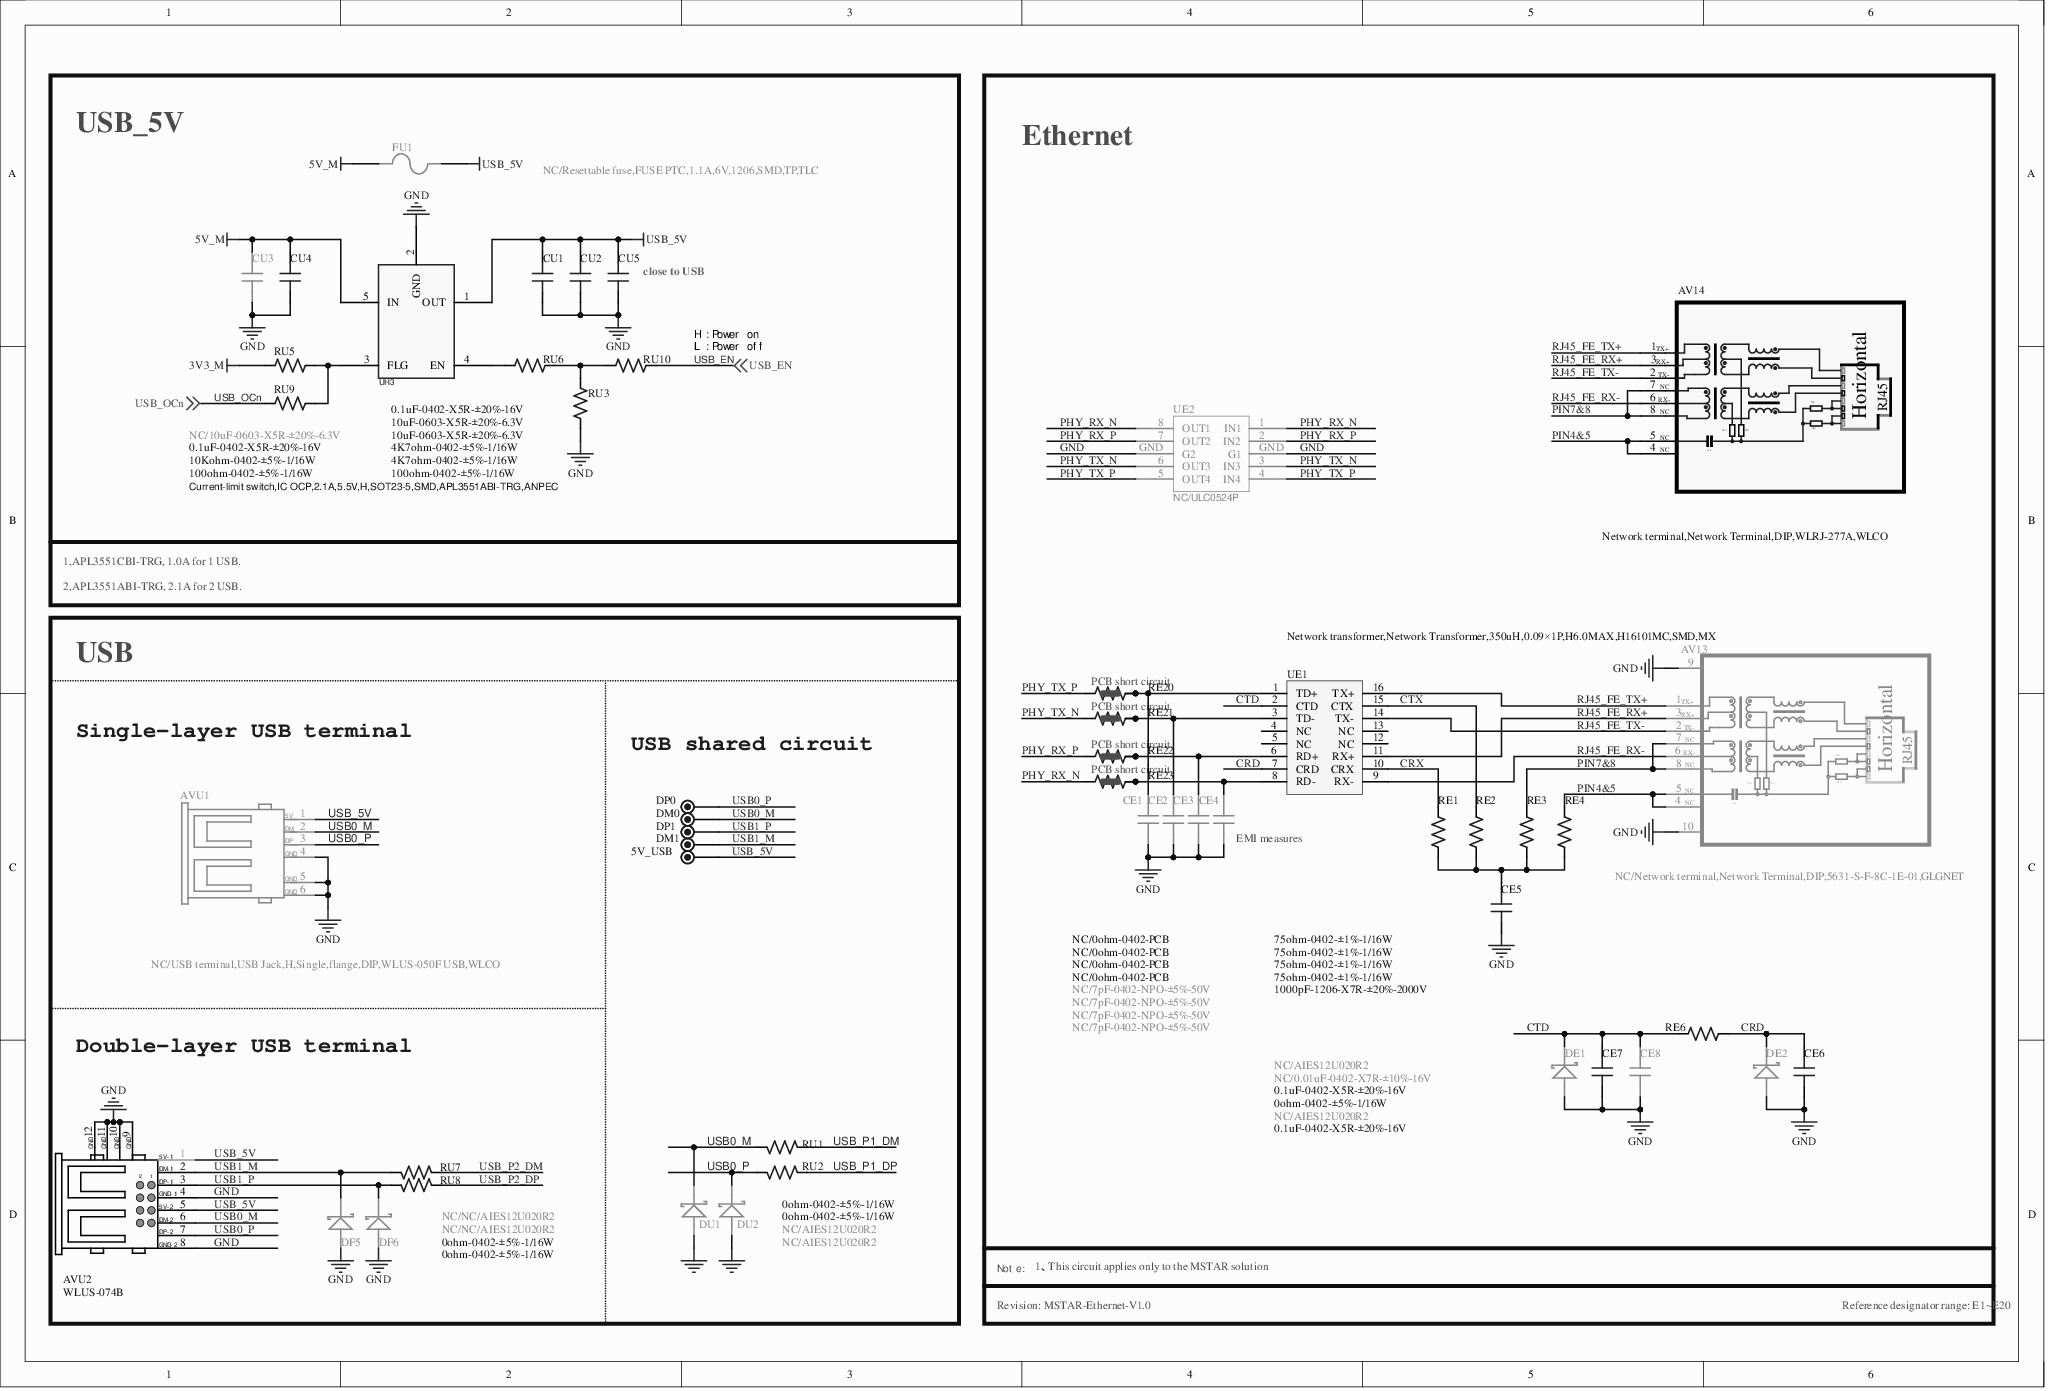
[diagram p0: MISC86290-16.SchDoc]
# Altium project MISC86290.PrjPcb (part 12 of 13)

## Sheet MISC86290-16.SchDoc
size 411 x 279 mm

### Parts
5V_USB  TEST  [TP]  (value not drawn)
AV13  NC/Network terminal,Network Terminal,DIP,5631-S-F-8C-1E-01,GLGNET  [RJ45U-D-5]
AV14  Network terminal,Network Terminal,DIP,WLRJ-277A,WLCO  [RJ45U-D-14]
AVU1  NC/USB terminal,USB Jack,H,Single,flange,DIP,WLUS-050F USB,WLCO  [USB1-HD-2]
AVU2  WLUS-074B  [USB2-HD-1]
CE1  NC/7pF-0402-NPO-±5%-50V  [C0402]
CE2  NC/7pF-0402-NPO-±5%-50V  [C0402]
CE3  NC/7pF-0402-NPO-±5%-50V  [C0402]
CE4  NC/7pF-0402-NPO-±5%-50V  [C0402]
CE5  1000pF-1206-X7R-±20%-2000V  [C1206]
CE6  0.1uF-0402-X5R-±20%-16V  [C0402]
CE7  0.1uF-0402-X5R-±20%-16V  [C0402]
CE8  NC/0.01uF-0402-X7R-±10%-16V  [C0402]
CU1  0.1uF-0402-X5R-±20%-16V  [C0402]
CU2  10uF-0603-X5R-±20%-6.3V  [C0603]
CU3  NC/10uF-0603-X5R-±20%-6.3V  [C0603]
CU4  0.1uF-0402-X5R-±20%-16V  [C0402]
CU5  10uF-0603-X5R-±20%-6.3V  [C0603]
DE1  NC/AIES12U020R2  [DIODE-S0402]
DE2  NC/AIES12U020R2  [DIODE-S0402]
DF5  NC/NC/AIES12U020R2  [DIODE-S0402]
DF6  NC/NC/AIES12U020R2  [DIODE-S0402]
DM0  TEST  [TP]  (value not drawn)
DM1  TEST  [TP]  (value not drawn)
DP0  TEST  [TP]  (value not drawn)
DP1  TEST  [TP]  (value not drawn)
DU1  NC/AIES12U020R2  [DIODE-S0402]
DU2  NC/AIES12U020R2  [DIODE-S0402]
FU1  NC/Resettable fuse,FUSE PTC,1.1A,6V,1206,SMD,TP,TLC  [FUSE1.1A-S]
RE1  75ohm-0402-±1%-1/16W  [R0402]
RE2  75ohm-0402-±1%-1/16W  [R0402]
RE3  75ohm-0402-±1%-1/16W  [R0402]
RE4  75ohm-0402-±1%-1/16W  [R0402]
RE6  0ohm-0402-±5%-1/16W  [R0402]
RE20  NC/0ohm-0402-PCB  [R0402SC]
RE21  NC/0ohm-0402-PCB  [R0402SC]
RE22  NC/0ohm-0402-PCB  [R0402SC]
RE23  NC/0ohm-0402-PCB  [R0402SC]
RU1  0ohm-0402-±5%-1/16W  [R0402]
RU2  0ohm-0402-±5%-1/16W  [R0402]
RU3  4K7ohm-0402-±5%-1/16W  [R0402]
RU5  10Kohm-0402-±5%-1/16W  [R0402]
RU6  4K7ohm-0402-±5%-1/16W  [R0402]
RU7  0ohm-0402-±5%-1/16W  [R0402]
RU8  0ohm-0402-±5%-1/16W  [R0402]
RU9  100ohm-0402-±5%-1/16W  [R0402]
RU10  100ohm-0402-±5%-1/16W  [R0402]
UE1  Network transformer,Network Transformer,350uH,0.09×1P,H6.0MAX,H16101MC,SMD,MX  [SOP16/1.27-2]
UE2  NC/ULC0524P  [RCL0524P]
UH3  Current-limit switch,IC OCP,2.1A,5.5V,H,SOT23-5,SMD,APL3551ABI-TRG,ANPEC  [SOT-23-5]

### Blocks framed on the sheet
USB_5V: CU1-CU5 FU1 RU3 RU5 RU6 RU9 RU10 UH3
Ethernet: AV13 AV14 CE1-CE8 DE1 DE2 RE1-RE4 RE6 RE20-RE23 UE1 UE2
USB: 5V_USB AVU1 AVU2 DF5 DF6 DM0 DM1 DP0 DP1 DU1 DU2 RU1 RU2 RU7 RU8

### Nets
3V3_M: RU5.1
5V_M: CU3.2 CU4.2 FU1.1 UH3.5(IN)
GND: AV13.9 AV13.10 AVU1.4 AVU1.5 AVU1.6 AVU2.4 AVU2.8 AVU2.9 AVU2.10 AVU2.11 AVU2.12 CE1.1 CE2.1 CE3.1 CE4.1 CE5.2 CE6.2 CE7.1 CE8.1 CU1.2 CU2.2 CU3.1 CU4.1 CU5.2 DE1.A DE2.A DF5.A DF6.A DU1.A DU2.A RU3.2 UE2.GND(G1) UH3.2(GND)
USB_5V: 5V_USB.1 AVU1.1 AVU2.1 AVU2.5 CU1.1 CU2.1 CU5.1 FU1.2 UH3.1(OUT)
CRD: CE6.1 DE2.K RE6.2 UE1.7(CRD)
CRX: RE1.2 UE1.10(CRX)
CTD: CE7.2 CE8.2 DE1.K RE6.1 UE1.2(CTD)
CTX: RE2.2 UE1.15(CTX)
PHY_RX_N: RE23.1 UE2.1(IN1) UE2.8(OUT1)
PHY_RX_P: RE22.1 UE2.2(IN2) UE2.7(OUT2)
PHY_TX_N: RE21.1 UE2.3(IN3) UE2.6(OUT3)
PHY_TX_P: RE20.1 UE2.4(IN4) UE2.5(OUT4)
PIN4&5: AV13.4 AV13.5 AV14.4 AV14.5 RE4.2
PIN7&8: AV13.7 AV13.8 AV14.7 AV14.8 RE3.2
RJ45_FE_RX+: AV13.3 AV14.3 UE1.11(RX+)
RJ45_FE_RX-: AV13.6 AV14.6 UE1.9(RX-)
RJ45_FE_TX+: AV13.1 AV14.1 UE1.16(TX+)
RJ45_FE_TX-: AV13.2 AV14.2 UE1.14(TX-)
USB0_M: AVU1.2 AVU2.6 DM0.1 DU1.K RU1.2
USB0_P: AVU1.3 AVU2.7 DP0.1 DU2.K RU2.2
USB1_M: AVU2.2 DF5.K DM1.1 RU7.2
USB1_P: AVU2.3 DF6.K DP1.1 RU8.2
USB_EN: RU10.2 ; off-sheet USB_EN
USB_OCn: RU9.1 ; off-sheet USB_OCn
USB_P1_DM: RU1.1
USB_P1_DP: RU2.1
USB_P2_DM: RU7.1
USB_P2_DP: RU8.1
NetCE1_2: CE1.2 RE20.2 RE20.3 UE1.1(TD+)
NetCE2_2: CE2.2 RE21.2 RE21.3 UE1.3(TD-)
NetCE3_2: CE3.2 RE22.2 RE22.3 UE1.6(RD+)
NetCE4_2: CE4.2 RE23.2 RE23.3 UE1.8(RD-)
NetCE5_1: CE5.1 RE1.1 RE2.1 RE3.1 RE4.1
NetRU3_1: RU3.1 RU6.1 RU10.1
NetRU5_2: RU5.2 RU9.2 UH3.3(FLG)
NetRU6_2: RU6.2 UH3.4(EN)

Not connected (* = marked no-connect by the designer): UE1 4(NC)* 5(NC)* 12(NC)* 13(NC)*

### Notes on the sheet
- (near CU5) close to USB
- H :Power on
- (near RU10) L :Power off
- 1,APL3551CBI-TRG, 1.0A for 1 USB.
- 2,APL3551ABI-TRG, 2.1A for 2 USB.
- Single-layer USB terminal
- USB shared circuit
- (near CE4) EMI measures
- Double-layer USB terminal
- Note:
- 1、This circuit applies only to the MSTAR solution
- Revision: MSTAR-Ethernet-V1.0
- Reference designator range: E1~E20

### Library data of the parts
AV13 = XXX.XXX.0002342: Network terminal,Network Terminal,DIP,5631-S-F-8C-1E-01,GLGNET-DLMI
AV14 = XXX.XXX.0002262: Network terminal,Network Terminal,DIP,41238-01G051,GLGNET-DLMI
AVU1 = USB-042M-002DP-DLMI-USB: CN-USB-#-#-#
AVU2 = USB-A/F-90°-DLMI-USB: CN-USB-double layer-#-#
CE1-CE4 = 7pF-0402-NPO-±5%-50V-D
CE5 = 1000pF-1206-X7R-±20%-2000V-D
CE6 CE7 CU1 = 0.1uF-0402-X5R-±20%-16V-D
CE8 = 0.01uF-0402-X7R-±10%-16V-D
CU2 CU3 CU5 = 10uF-0603-X5R-±20%-6.3V-D
CU4 = 0.1uF-0402-X7R-±10%-16V-D
DE1 DE2 DF5 DF6 DU1 DU2 = AIES12U020R2-D
FU1 = NSMD110(1206-1.1A)-D
RE1-RE4 = 75ohm-0402-±1%-1/16W-D
RE6 = 0ohm-0402-±5%-1/16W-D
RE20-RE23 = 0ohm-0402-PCB-D
RU1 RU2 RU7 RU8 = 5R1ohm-0402-±5%-1/16W-D
RU3 RU6 = 4K7ohm-0402-±5%-1/16W-D
RU5 RU9 RU10 = 10Kohm-0402-±5%-1/16W-D
UE1 = H16101MC-D
UE2 = ULC0524P-D: RCLAMP0524J
UH3 = AP2171WG-7-D

## Sheet MISC86290-17.SchDoc
size 406 x 325 mm
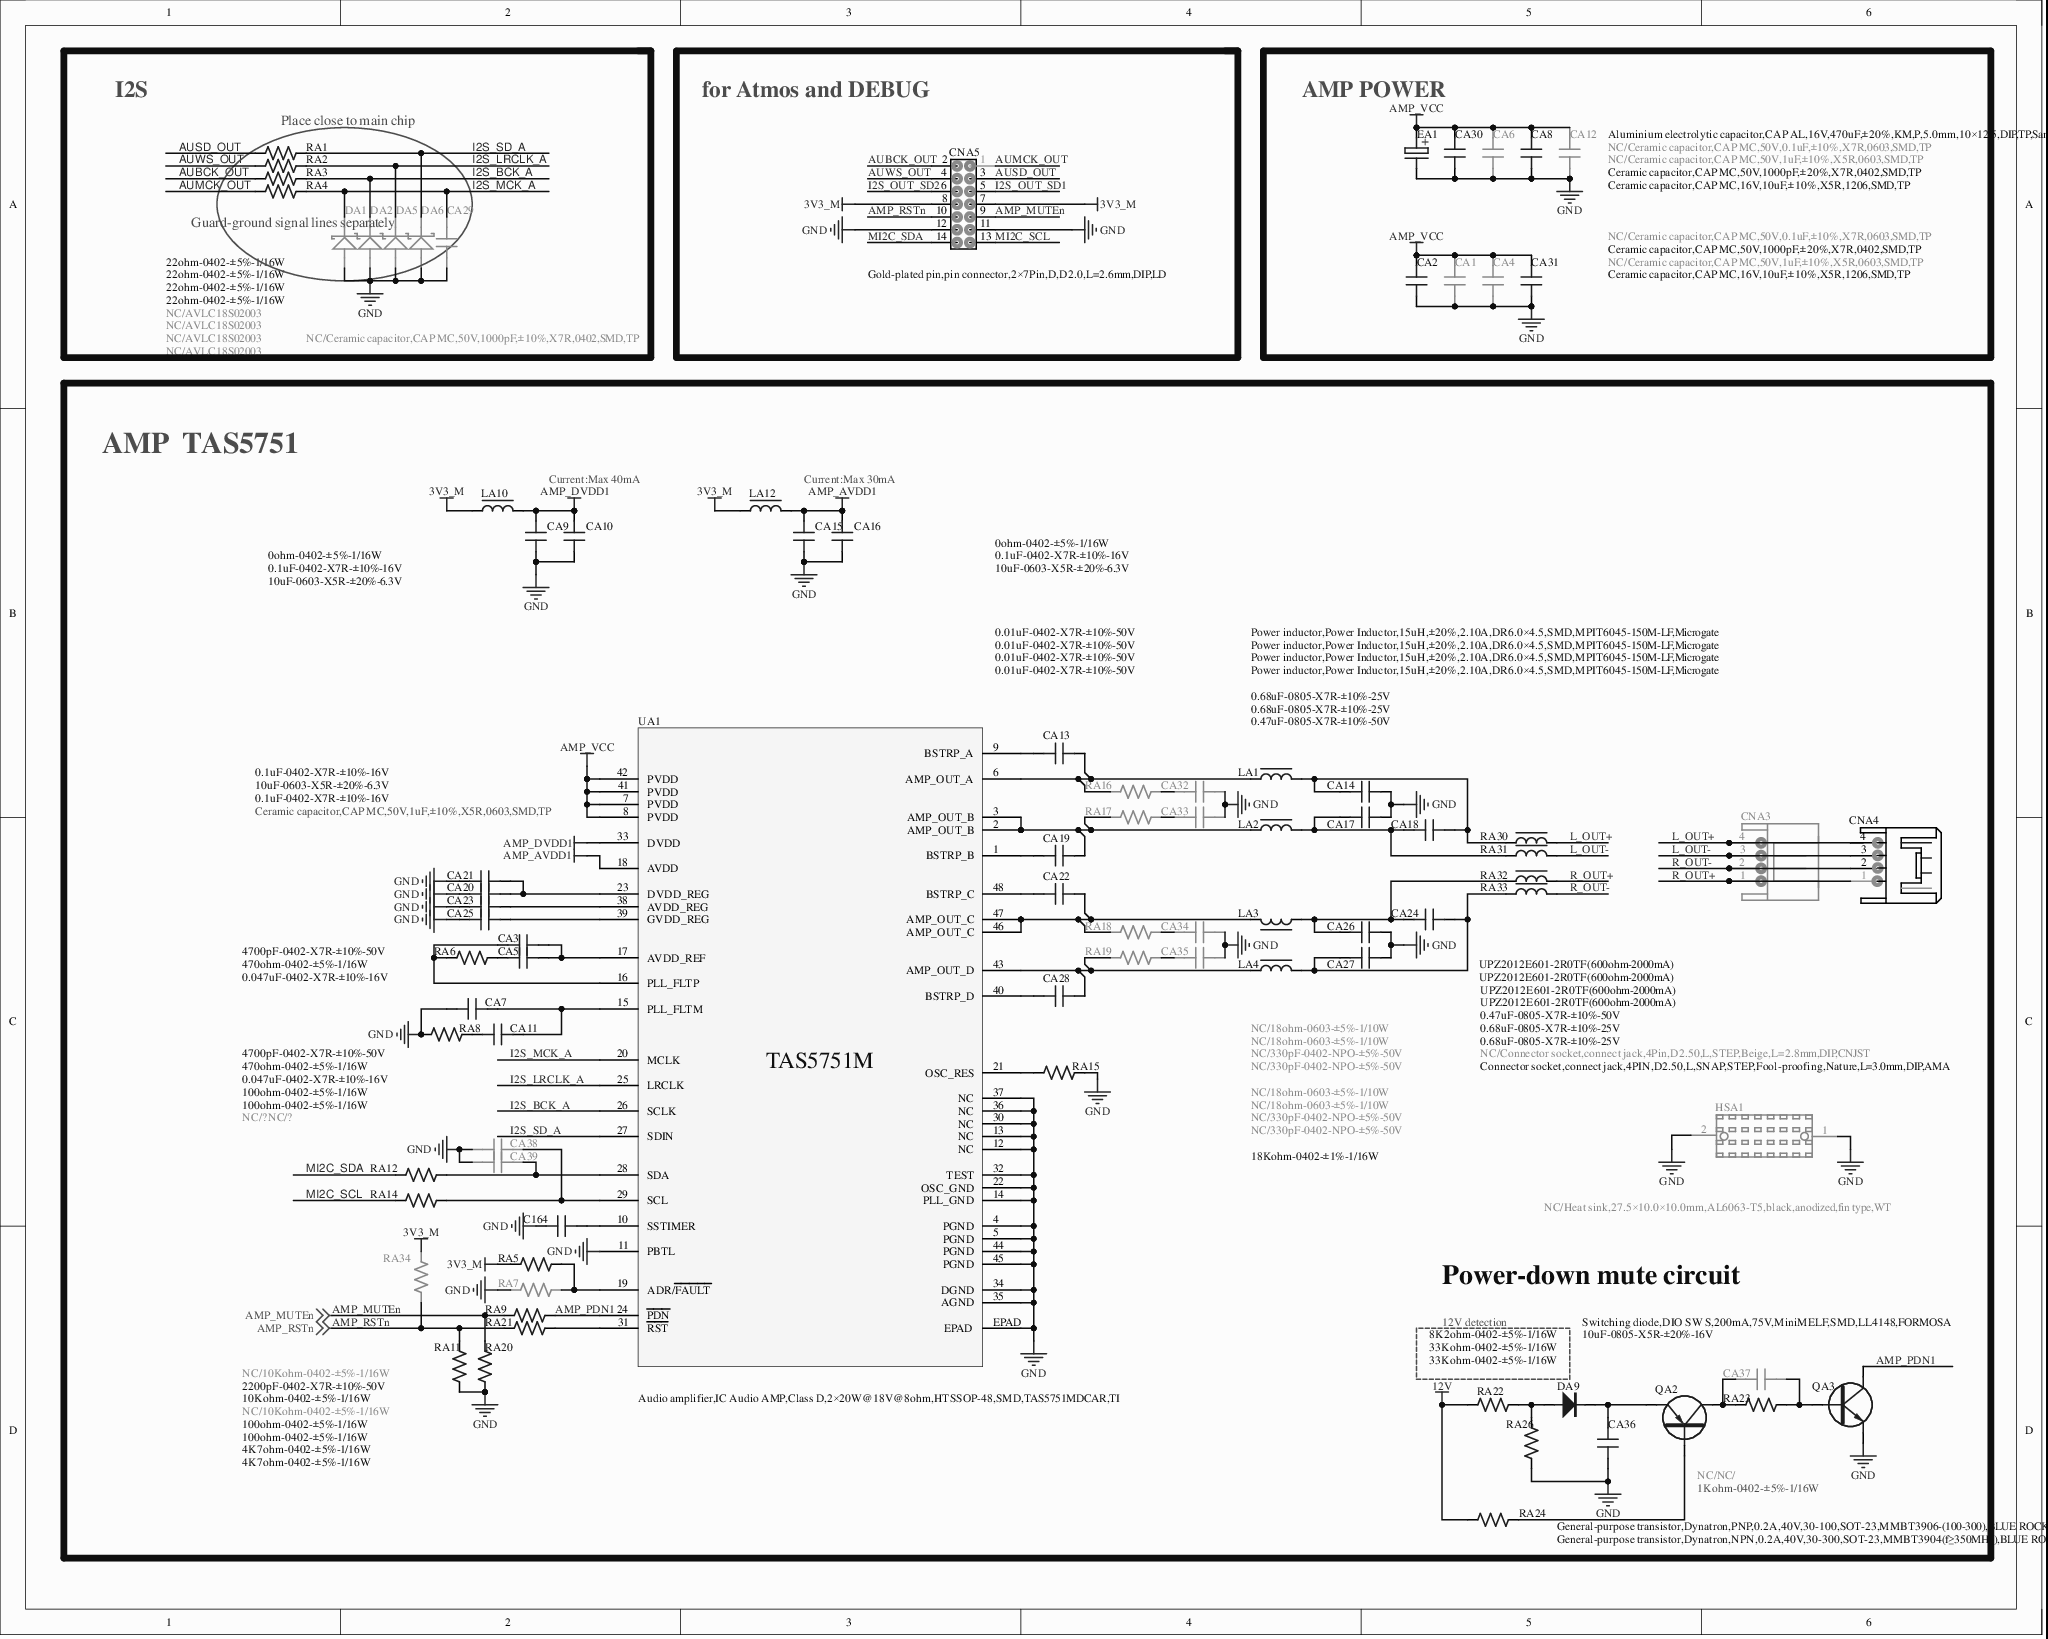
[diagram p1: MISC86290-17.SchDoc]

### Parts
C164  2200pF-0402-X7R-±10%-50V  [C0402]
CA1  NC/Ceramic capacitor,CAP MC,50V,0.1uF,±10%,X7R,0603,SMD,TP  [C0603]
CA2  Ceramic capacitor,CAP MC,50V,1000pF,±20%,X7R,0402,SMD,TP  [C0402]
CA3  4700pF-0402-X7R-±10%-50V  [C0402]
CA4  NC/Ceramic capacitor,CAP MC,50V,1uF,±10%,X5R,0603,SMD,TP  [C0603]
CA5  0.047uF-0402-X7R-±10%-16V  [C0402]
CA6  NC/Ceramic capacitor,CAP MC,50V,0.1uF,±10%,X7R,0603,SMD,TP  [C0603]
CA7  4700pF-0402-X7R-±10%-50V  [C0402]
CA8  Ceramic capacitor,CAP MC,50V,1000pF,±20%,X7R,0402,SMD,TP  [C0402]
CA9  0.1uF-0402-X7R-±10%-16V  [C0402]
CA10  10uF-0603-X5R-±20%-6.3V  [C0603]
CA11  0.047uF-0402-X7R-±10%-16V  [C0402]
CA12  NC/Ceramic capacitor,CAP MC,50V,1uF,±10%,X5R,0603,SMD,TP  [C0603]
CA13  0.01uF-0402-X7R-±10%-50V  [C0402]
CA14  0.68uF-0805-X7R-±10%-25V  [C0805]
CA15  0.1uF-0402-X7R-±10%-16V  [C0402]
CA16  10uF-0603-X5R-±20%-6.3V  [C0603]
CA17  0.68uF-0805-X7R-±10%-25V  [C0805]
CA18  0.47uF-0805-X7R-±10%-50V  [C0805]
CA19  0.01uF-0402-X7R-±10%-50V  [C0402]
CA20  0.1uF-0402-X7R-±10%-16V  [C0402]
CA21  10uF-0603-X5R-±20%-6.3V  [C0603]
CA22  0.01uF-0402-X7R-±10%-50V  [C0402]
CA23  0.1uF-0402-X7R-±10%-16V  [C0402]
CA24  0.47uF-0805-X7R-±10%-50V  [C0805]
CA25  Ceramic capacitor,CAP MC,50V,1uF,±10%,X5R,0603,SMD,TP  [C0603]
CA26  0.68uF-0805-X7R-±10%-25V  [C0805]
CA27  0.68uF-0805-X7R-±10%-25V  [C0805]
CA28  0.01uF-0402-X7R-±10%-50V  [C0402]
CA29  NC/Ceramic capacitor,CAP MC,50V,1000pF,±10%,X7R,0402,SMD,TP  [C0402]
CA30  Ceramic capacitor,CAP MC,16V,10uF,±10%,X5R,1206,SMD,TP  [C1206]
CA31  Ceramic capacitor,CAP MC,16V,10uF,±10%,X5R,1206,SMD,TP  [C1206]
CA32  NC/330pF-0402-NPO-±5%-50V  [C0402]
CA33  NC/330pF-0402-NPO-±5%-50V  [C0402]
CA34  NC/330pF-0402-NPO-±5%-50V  [C0402]
CA35  NC/330pF-0402-NPO-±5%-50V  [C0402]
CA36  10uF-0805-X5R-±20%-16V  [C0805]
CA37  NC/NC/  [C0402]
CA38  NC/?  [C0402]
CA39  NC/?  [C0402]
CNA3  NC/Connector socket,connect jack,4Pin,D2.50,L,STEP,Beige,L=2.8mm,DIP,CNJST  [SIP4H/2.5D-4]
CNA4  Connector socket,connect jack,4PIN,D2.50,L,SNAP,STEP,Fool-proofing,Nature,L=3.0mm,DIP,AMA  [SIP4H/2.5D-7]
CNA5  Gold-plated pin,pin connector,2×7Pin,D,D2.0,L=2.6mm,DIP,LD  [SIP2*7/2.0D]
DA1  NC/AVLC18S02003  [DIODE-S0402]
DA2  NC/AVLC18S02003  [DIODE-S0402]
DA5  NC/AVLC18S02003  [DIODE-S0402]
DA6  NC/AVLC18S02003  [DIODE-S0402]
DA9  Switching diode,DIO SW S,200mA,75V,MiniMELF,SMD,LL4148,FORMOSA  [DIODE-S0805]
EA1  Aluminium electrolytic capacitor,CAP AL,16V,470uF,±20%,KM,P,5.0mm,10×12.5,DIP,TP,Samxon  [EC(10*13)-V-5.0-1]
HSA1  NC/Heat sink,27.5×10.0×10.0mm,AL6063-T5,black,anodized,fin type,WT  [HS(27*10*10)-1]
LA1  Power inductor,Power Inductor,15uH,±20%,2.10A,DR6.0×4.5,SMD,MPIT6045-150M-LF,Microgate  [L(6.0*4.5)-S]
LA2  Power inductor,Power Inductor,15uH,±20%,2.10A,DR6.0×4.5,SMD,MPIT6045-150M-LF,Microgate  [L(6.0*4.5)-S]
LA3  Power inductor,Power Inductor,15uH,±20%,2.10A,DR6.0×4.5,SMD,MPIT6045-150M-LF,Microgate  [L(6.0*4.5)-S]
LA4  Power inductor,Power Inductor,15uH,±20%,2.10A,DR6.0×4.5,SMD,MPIT6045-150M-LF,Microgate  [L(6.0*4.5)-S]
LA10  0ohm-0402-±5%-1/16W  [L0402]
LA12  0ohm-0402-±5%-1/16W  [L0402]
QA2  General-purpose transistor,Dynatron,PNP,0.2A,40V,30-100,SOT-23,MMBT3906-(100-300),BLUE ROCKET  [SOT-23]
QA3  General-purpose transistor,Dynatron,NPN,0.2A,40V,30-300,SOT-23,MMBT3904(f≥350MHz),BLUE ROCKET  [SOT-23]
RA1  22ohm-0402-±5%-1/16W  [R0402]
RA2  22ohm-0402-±5%-1/16W  [R0402]
RA3  22ohm-0402-±5%-1/16W  [R0402]
RA4  22ohm-0402-±5%-1/16W  [R0402]
RA5  10Kohm-0402-±5%-1/16W  [R0402]
RA6  470ohm-0402-±5%-1/16W  [R0402]
RA7  NC/10Kohm-0402-±5%-1/16W  [R0402]
RA8  470ohm-0402-±5%-1/16W  [R0402]
RA9  100ohm-0402-±5%-1/16W  [R0402]
RA11  4K7ohm-0402-±5%-1/16W  [R0402]
RA12  100ohm-0402-±5%-1/16W  [R0402]
RA14  100ohm-0402-±5%-1/16W  [R0402]
RA15  18Kohm-0402-±1%-1/16W  [R0402]
RA16  NC/18ohm-0603-±5%-1/10W  [R0603]
RA17  NC/18ohm-0603-±5%-1/10W  [R0603]
RA18  NC/18ohm-0603-±5%-1/10W  [R0603]
RA19  NC/18ohm-0603-±5%-1/10W  [R0603]
RA20  4K7ohm-0402-±5%-1/16W  [R0402]
RA21  100ohm-0402-±5%-1/16W  [R0402]
RA22  8K2ohm-0402-±5%-1/16W  [R0402]
RA23  1Kohm-0402-±5%-1/16W  [R0402]
RA24  33Kohm-0402-±5%-1/16W  [R0402]
RA26  33Kohm-0402-±5%-1/16W  [R0402]
RA30  UPZ2012E601-2R0TF(600ohm-2000mA)  [L0805]
RA31  UPZ2012E601-2R0TF(600ohm-2000mA)  [L0805]
RA32  UPZ2012E601-2R0TF(600ohm-2000mA)  [L0805]
RA33  UPZ2012E601-2R0TF(600ohm-2000mA)  [L0805]
RA34  NC/10Kohm-0402-±5%-1/16W  [R0402]
UA1  Audio amplifier,IC Audio AMP,Class D,2×20W@18V@8ohm,HTSSOP-48,SMD,TAS5751MDCAR,TI  [SOP48/0.5-2]

### Blocks framed on the sheet
AMP POWER: CA1 CA2 CA4 CA6 CA8 CA12 CA30 CA31 EA1
AMP  TAS5751: C164 CA3 CA5 CA7 CA9-CA11 CA13-CA28 CA32-CA39 CNA3 CNA4 DA9 HSA1 LA1-LA4 LA10 LA12 QA2 QA3 RA5-RA9 RA11 RA12 RA14-RA24 RA26 RA30-RA34 UA1

### Nets
3V3_M: CNA5.7 CNA5.8 LA10.1 LA12.1 RA5.1 RA34.1
12V: RA22.1 RA24.2
AMP_AVDD1: CA15.2 CA16.2 LA12.2 UA1.18(AVDD)
AMP_DVDD1: CA9.2 CA10.2 LA10.2 UA1.33(DVDD)
AMP_VCC: CA1.2 CA2.2 CA4.2 CA6.2 CA8.2 CA12.2 CA30.2 CA31.2 EA1.1 UA1.7(PVDD) UA1.8(PVDD) UA1.41(PVDD) UA1.42(PVDD)
GND: C164.2 CA1.1 CA2.1 CA4.1 CA6.1 CA7.1 CA8.1 CA9.1 CA10.1 CA12.1 CA14.2 CA15.1 CA16.1 CA17.2 CA20.2 CA21.1 CA23.2 CA25.2 CA26.2 CA27.2 CA29.1 CA30.1 CA31.1 CA32.2 CA33.2 CA34.2 CA35.2 CA36.1 CA38.1 CA39.1 CNA5.11 CNA5.12 DA1.A DA2.A DA5.A DA6.A EA1.2 HSA1.1(GND) HSA1.2(GND) QA3.E RA7.2 RA8.1 RA11.1 RA15.2 RA20.1 RA26.1 UA1.4(PGND) UA1.5(PGND) UA1.11(PBTL) UA1.12(NC) UA1.13(NC) UA1.14(PLL_GND) UA1.22(OSC_GND) UA1.30(NC) UA1.32(TEST) UA1.34(DGND) UA1.35(AGND) UA1.36(NC) UA1.37(NC) UA1.44(PGND) UA1.45(PGND) UA1.EPAD
AMP_MUTEn: CNA5.9 RA9.2 RA20.2 ; off-sheet AMP_MUTEn
AMP_PDN1: QA3.C RA9.1 UA1.24(~{PDN})
AMP_RSTn: CNA5.10 RA11.2 RA21.1 RA34.2 ; off-sheet AMP_RSTn
AUBCK_OUT: CNA5.2 RA3.1
AUMCK_OUT: CNA5.1 RA4.1
AUSD_OUT: CNA5.3 RA1.1
AUWS_OUT: CNA5.4 RA2.1
I2S_BCK_A: DA2.K RA3.2 UA1.26(SCLK)
I2S_LRCLK_A: DA5.K RA2.2 UA1.25(LRCLK)
I2S_MCK_A: CA29.2 DA1.K RA4.2 UA1.20(MCLK)
I2S_OUT_SD1: CNA5.5
I2S_OUT_SD2: CNA5.6
I2S_SD_A: DA6.K RA1.2 UA1.27(SDIN)
L_OUT+: CNA3.4 CNA4.4 RA30.2
L_OUT-: CNA3.3 CNA4.3 RA31.2
MI2C_SCL: CNA5.13 RA14.1
MI2C_SDA: CNA5.14 RA12.1
R_OUT+: CNA3.1 CNA4.1 RA32.2
R_OUT-: CNA3.2 CNA4.2 RA33.2
NetC164_1: C164.1 UA1.10(SSTIMER)
NetCA3_1: CA3.1 RA6.1 UA1.16(PLL_FLTP)
NetCA3_2: CA3.2 CA5.2 UA1.17(AVDD_REF)
NetCA5_1: CA5.1 RA6.2
NetCA7_2: CA7.2 CA11.2 UA1.15(PLL_FLTM)
NetCA11_1: CA11.1 RA8.2
NetCA13_1: CA13.1 UA1.9(BSTRP_A)
NetCA13_2: CA13.2 LA1.1 RA16.1 UA1.6(AMP_OUT_A)
NetCA14_1: CA14.1 CA18.2 LA1.2 RA30.1
NetCA17_1: CA17.1 CA18.1 LA2.2 RA31.1
NetCA19_1: CA19.1 UA1.1(BSTRP_B)
NetCA19_2: CA19.2 LA2.1 RA17.1 UA1.2(AMP_OUT_B) UA1.3(AMP_OUT_B)
NetCA20_1: CA20.1 CA21.2 UA1.23(DVDD_REG)
NetCA22_1: CA22.1 UA1.48(BSTRP_C)
NetCA22_2: CA22.2 LA3.2 RA18.1 UA1.46(AMP_OUT_C) UA1.47(AMP_OUT_C)
NetCA23_1: CA23.1 UA1.38(AVDD_REG)
NetCA24_1: CA24.1 CA26.1 LA3.1 RA32.1
NetCA24_2: CA24.2 CA27.1 LA4.2 RA33.1
NetCA25_1: CA25.1 UA1.39(GVDD_REG)
NetCA28_1: CA28.1 UA1.40(BSTRP_D)
NetCA28_2: CA28.2 LA4.1 RA19.1 UA1.43(AMP_OUT_D)
NetCA32_1: CA32.1 RA16.2
NetCA33_1: CA33.1 RA17.2
NetCA34_1: CA34.1 RA18.2
NetCA35_1: CA35.1 RA19.2
NetCA36_2: CA36.2 DA9.K QA2.E
NetCA37_1: CA37.1 QA2.C RA23.1
NetCA37_2: CA37.2 QA3.B RA23.2
NetCA38_2: CA38.2 RA14.2 UA1.29(SCL)
NetCA39_2: CA39.2 RA12.2 UA1.28(SDA)
NetDA9_A: DA9.A RA22.2 RA26.2
NetQA2_B: QA2.B RA24.1
NetRA5_2: RA5.2 RA7.1 UA1.19(ADR/~{FAULT})
NetRA15_1: RA15.1 UA1.21(OSC_RES)
NetRA21_2: RA21.2 UA1.31(~{RST})

### Notes on the sheet
- I2S
- Place close to main chip
- for Atmos and DEBUG
- Guard-ground signal lines separately
- Current:Max 40mA
- Current:Max 30mA
- 12V detection
- Power-down mute circuit

### Library data of the parts
C164 = 2200pF-0402-X7R-±10%-50V-D
CA1 CA6 = 004.003.0000044-D: Ceramic capacitor,CAP MC,50V,0.1uF,±10%,X7R,0603,SMD,TP-D
CA2 CA8 CA29 = 004.003.0000503-D: Ceramic capacitor,CAP MC,50V,1000pF,±10%,X7R,0402,SMD,TP-D
CA3 CA7 = 4700pF-0402-X7R-±10%-50V-D
CA4 CA12 CA25 = 004.003.0000667-D: Ceramic capacitor,CAP MC,50V,1uF,±10%,X5R,0603,SMD,TP-D
CA5 CA11 CA38 CA39 = 0.047uF-0402-X7R-±10%-16V-D
CA9 CA15 CA20 CA23 = 0.1uF-0402-X5R-±20%-16V-D
CA10 CA16 CA21 = 10uF-0603-X5R-±20%-6.3V-D
CA13 CA19 CA22 CA28 = 0.01uF-0402-X7R-±10%-50V-D
CA14 CA17 CA26 CA27 = 0.68uF-0805-X7R-±10%-25V-D
CA18 CA24 = 0.47uF-0805-X7R-±10%-50V-D
CA30 CA31 = 004.003.0000956-D: Ceramic capacitor,CAP MC,50V,10uF,±10%,X5R,1206,SMD,TP-D
CA32-CA35 = 330pF-0402-NPO-±5%-50V-D
CA36 = 10uF-0805-X5R-±20%-16V-D
CA37 = 1uF-0402-X5R-±20%-6.3V-D
CNA3 = XXX.XXX.0000762-DLMI: Connector socket,connect jack,4Pin,D2.50,L,STEP,Beige,L=2.8mm,DIP,CNJST-DLMI
CNA4 = XXX.XXX.0001836-DLMI: Connector socket,connect jack,4PIN,D2.50,L,SNAP,STEP,Fool-proofing,Nature,L=3.0mm,DIP,AMA-DLMI
CNA5 = XXX.XXX.0002239-DHMI: Gold-plated pin,pin connector,2×7Pin,D,D2.0,L=2.6mm,DIP,LD-DHMI
DA1 DA2 DA5 DA6 = AVLC18S02003-D
DA9 = PMLL4148L-F-D
EA1 = 004.003.0000454-DHMI: Aluminium electrolytic capacitor,CAP AL,35V,470uF,±20%,RK,P,5.0mm,10×13,DIP,TP,XL-DHMI
HSA1 = 27*10*10-HS: HS-natural colour
LA1-LA4 = MPIT6045-150M-LF-D
LA10 LA12 = FCM1005KF-121T06(120ohm-500mA)-D
QA2 = 3CG3906M-D: Q-PNP-#-#-#
QA3 = LMBT3904LT1G-D-NPN: Q-NPN-#-#-#
RA1-RA4 = 22ohm-0402-±5%-1/16W-D
RA5 RA7 RA34 = 10Kohm-0402-±5%-1/16W-D
RA6 RA8 RA12 RA14 = 470ohm-0402-±5%-1/16W-D
RA9 = 100ohm-0402-±5%-1/16W-D
RA11 RA20 = 4K7ohm-0402-±5%-1/16W-D
RA15 = 18Kohm-0402-±1%-1/16W-D
RA16-RA19 = 18ohm-0603-±5%-1/10W-D
RA21 RA23 = 1Kohm-0402-±5%-1/16W-D
RA22 = 8K2ohm-0402-±5%-1/16W-D
RA24 RA26 = 33Kohm-0402-±5%-1/16W-D
RA30-RA33 = 300ohm-2500mA-0805-D
UA1 = PKG-002027/P000038588: Audio amplifier,IC Audio AMP,Class D,2×20W@18.0V@8ohm,HTSSOP48,SMD,TAS5751MDCAR,TI-D

## Sheet MISC86290-18.SchDoc
size 431 x 228 mm
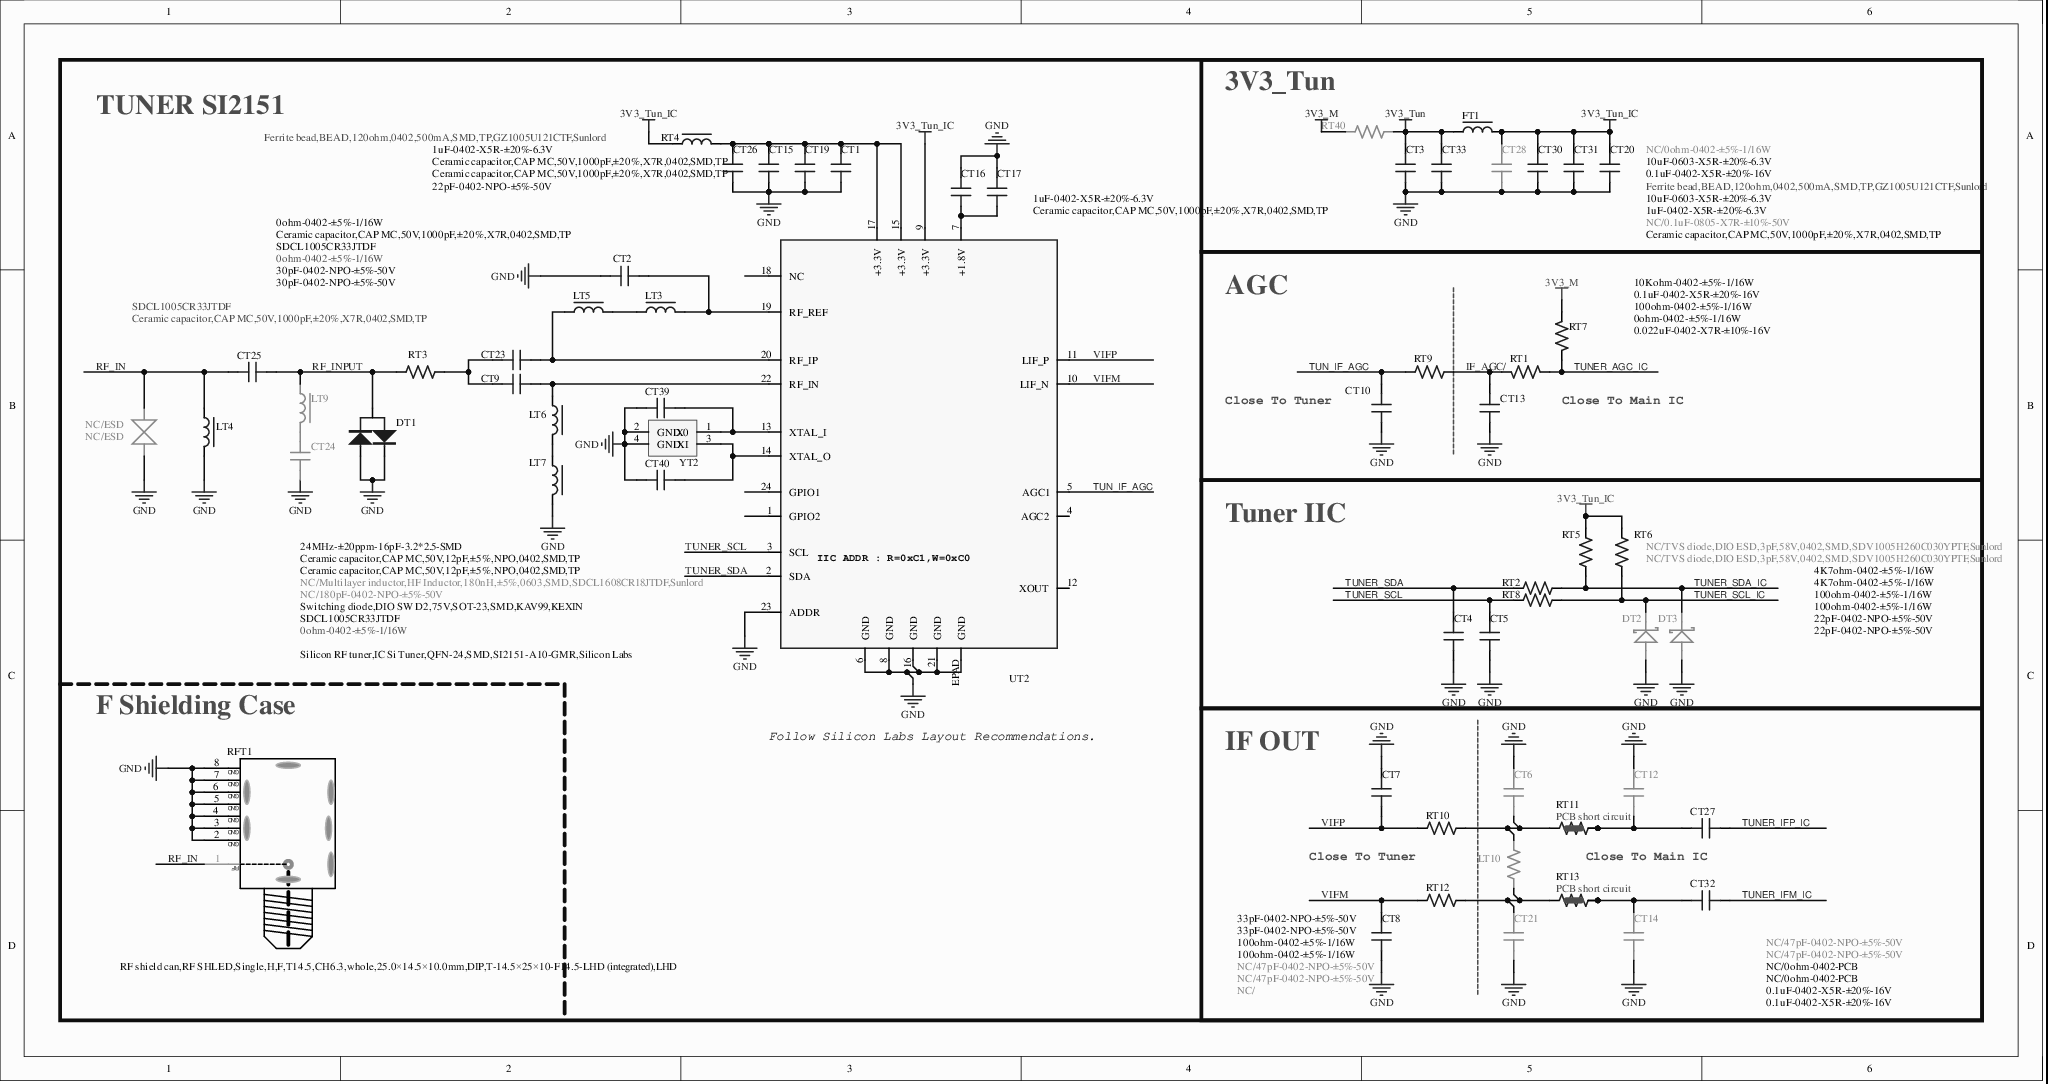
[diagram p2: MISC86290-18.SchDoc]

### Parts
CT1  Ceramic capacitor,CAP MC,50V,1000pF,±20%,X7R,0402,SMD,TP  [C0402]
CT2  Ceramic capacitor,CAP MC,50V,1000pF,±20%,X7R,0402,SMD,TP  [C0402]
CT3  10uF-0603-X5R-±20%-6.3V  [C0603]
CT4  22pF-0402-NPO-±5%-50V  [C0402]
CT5  22pF-0402-NPO-±5%-50V  [C0402]
CT6  NC/47pF-0402-NPO-±5%-50V  [C0402]
CT7  33pF-0402-NPO-±5%-50V  [C0402]
CT8  33pF-0402-NPO-±5%-50V  [C0402]
CT9  30pF-0402-NPO-±5%-50V  [C0402]
CT10  0.1uF-0402-X5R-±20%-16V  [C0402]
CT12  NC/47pF-0402-NPO-±5%-50V  [C0402]
CT13  0.022uF-0402-X7R-±10%-16V  [C0402]
CT14  NC/47pF-0402-NPO-±5%-50V  [C0402]
CT15  1uF-0402-X5R-±20%-6.3V  [C0402]
CT16  1uF-0402-X5R-±20%-6.3V  [C0402]
CT17  Ceramic capacitor,CAP MC,50V,1000pF,±20%,X7R,0402,SMD,TP  [C0402]
CT19  Ceramic capacitor,CAP MC,50V,1000pF,±20%,X7R,0402,SMD,TP  [C0402]
CT20  Ceramic capacitor,CAP MC,50V,1000pF,±20%,X7R,0402,SMD,TP  [C0402]
CT21  NC/47pF-0402-NPO-±5%-50V  [C0402]
CT23  30pF-0402-NPO-±5%-50V  [C0402]
CT24  NC/180pF-0402-NPO-±5%-50V  [C0402]
CT25  Ceramic capacitor,CAP MC,50V,1000pF,±20%,X7R,0402,SMD,TP  [C0402]
CT26  22pF-0402-NPO-±5%-50V  [C0402]
CT27  0.1uF-0402-X5R-±20%-16V  [C0402]
CT28  NC/0.1uF-0805-X7R-±10%-50V  [C0805]
CT30  10uF-0603-X5R-±20%-6.3V  [C0603]
CT31  1uF-0402-X5R-±20%-6.3V  [C0402]
CT32  0.1uF-0402-X5R-±20%-16V  [C0402]
CT33  0.1uF-0402-X5R-±20%-16V  [C0402]
CT39  Ceramic capacitor,CAP MC,50V,12pF,±5%,NPO,0402,SMD,TP  [C0402]
CT40  Ceramic capacitor,CAP MC,50V,12pF,±5%,NPO,0402,SMD,TP  [C0402]
DT1  Switching diode,DIO SW D2,75V,SOT-23,SMD,KAV99,KEXIN  [SO-23]
DT2  NC/TVS diode,DIO ESD,3pF,58V,0402,SMD,SDV1005H260C030YPTF,Sunlord  [DIODE-S0402]
DT3  NC/TVS diode,DIO ESD,3pF,58V,0402,SMD,SDV1005H260C030YPTF,Sunlord  [DIODE-S0402]
FT1  Ferrite bead,BEAD,120ohm,0402,500mA,SMD,TP,GZ1005U121CTF,Sunlord  [L0402]
LT3  0ohm-0402-±5%-1/16W  [L0402]
LT4  SDCL1005CR33JTDF  [L0402]
LT5  SDCL1005CR33JTDF  [L0402]
LT6  SDCL1005CR33JTDF  [L0402]
LT7  0ohm-0402-±5%-1/16W  [L0402]
LT9  NC/Multilayer inductor,HF Inductor,180nH,±5%,0603,SMD,SDCL1608CR18JTDF,Sunlord  [L0603]
LT10  NC/  [R0402]
NC/ESD  NC/ESD  [ESD]
RFT1  RF shield can,RF SHLED,Single,H,F,T14.5,CH6.3,whole,25.0×14.5×10.0mm,DIP,T-14.5×25×10-F14.5-LHD (integrated),LHD  [T-14.5×25×10-F14.5-2]
RT1  0ohm-0402-±5%-1/16W  [R0402]
RT2  100ohm-0402-±5%-1/16W  [R0402]
RT3  0ohm-0402-±5%-1/16W  [R0402]
RT4  Ferrite bead,BEAD,120ohm,0402,500mA,SMD,TP,GZ1005U121CTF,Sunlord  [L0402]
RT5  4K7ohm-0402-±5%-1/16W  [R0402]
RT6  4K7ohm-0402-±5%-1/16W  [R0402]
RT7  10Kohm-0402-±5%-1/16W  [R0402]
RT8  100ohm-0402-±5%-1/16W  [R0402]
RT9  100ohm-0402-±5%-1/16W  [R0402]
RT10  100ohm-0402-±5%-1/16W  [R0402]
RT11  NC/0ohm-0402-PCB  [R0402SC]
RT12  100ohm-0402-±5%-1/16W  [R0402]
RT13  NC/0ohm-0402-PCB  [R0402SC]
RT40  NC/0ohm-0402-±5%-1/16W  [R0402]
UT2  Silicon RF tuner,IC Si Tuner,QFN-24,SMD,SI2151-A10-GMR,Silicon Labs  [QFN24/0.4-1]
YT2  24MHz-±20ppm-16pF-3.2*2.5-SMD  [XTAL-S-3]

### Blocks framed on the sheet
3V3_Tun: CT3 CT20 CT28 CT30 CT31 CT33 FT1 RT40
AGC: CT10 CT13 RT1 RT7 RT9
Tuner IIC: CT4 CT5 DT2 DT3 RT2 RT5 RT6 RT8
IF OUT: CT6-CT8 CT12 CT14 CT21 CT27 CT32 LT10 RT10-RT13

### Nets
3V3_M: RT7.2 RT40.1
3V3_Tun: CT3.2 CT33.2 FT1.1 RT40.2
3V3_Tun_IC: CT20.2 CT28.2 CT30.2 CT31.2 FT1.2 RT4.1 RT5.2 RT6.2 UT2.9(+3.3V)
GND: CT1.1 CT2.1 CT3.1 CT4.2 CT5.2 CT6.1 CT7.1 CT8.1 CT10.1 CT12.1 CT13.1 CT14.2 CT15.2 CT16.1 CT17.1 CT19.1 CT20.1 CT21.2 CT24.2 CT26.1 CT28.1 CT30.1 CT31.1 CT33.1 CT39.1 CT40.1 DT1.1 DT1.3 DT2.A DT3.A LT4.2 LT7.2 NC/ESD.1 RFT1.2 RFT1.3 RFT1.4 RFT1.5 RFT1.6 RFT1.7 RFT1.8 UT2.6(GND) UT2.8(GND) UT2.16(GND) UT2.21(GND) UT2.23(ADDR) UT2.EPAD(GND) YT2.2(GND) YT2.4(GND)
IF_AGC/: CT13.2 RT1.1 RT9.2
RF_IN: CT25.1 LT4.1 NC/ESD.2 RFT1.1
RF_INPUT: CT25.2 DT1.2 LT9.1 RT3.1
TUN_IF_AGC: CT10.2 RT9.1 UT2.5(AGC1)
TUNER_AGC_IC: RT1.2 RT7.1
TUNER_IFM_IC: CT32.2
TUNER_IFP_IC: CT27.1
TUNER_SCL: CT5.1 RT8.1 UT2.3(SCL)
TUNER_SCL_IC: DT2.K RT6.1 RT8.2
TUNER_SDA: CT4.1 RT2.1 UT2.2(SDA)
TUNER_SDA_IC: DT3.K RT2.2 RT5.1
VIFM: CT8.2 RT12.1 UT2.10(LIF_N)
VIFP: CT7.2 RT10.1 UT2.11(LIF_P)
NetCT1_2: CT1.2 CT15.1 CT19.2 CT26.2 RT4.2 UT2.15(+3.3V) UT2.17(+3.3V)
NetCT2_2: CT2.2 LT3.2 UT2.19(RF_REF)
NetCT6_2: CT6.2 LT10.1 RT10.2 RT11.1
NetCT9_1: CT9.1 LT6.1 UT2.22(RF_IN)
NetCT9_2: CT9.2 CT23.2 RT3.2
NetCT12_2: CT12.2 CT27.2 RT11.2 RT11.3
NetCT14_1: CT14.1 CT32.1 RT13.2 RT13.3
NetCT16_2: CT16.2 CT17.2 UT2.7(+1.8V)
NetCT21_1: CT21.1 LT10.2 RT12.2 RT13.1
NetCT23_1: CT23.1 LT5.1 UT2.20(RF_IP)
NetCT24_1: CT24.1 LT9.2
NetCT39_2: CT39.2 UT2.13(XTAL_I) YT2.1(X0)
NetCT40_2: CT40.2 UT2.14(XTAL_O) YT2.3(XI)
NetLT3_1: LT3.1 LT5.2
NetLT6_2: LT6.2 LT7.1

Not connected (* = marked no-connect by the designer): UT2 1(GPIO2)* 4(AGC2)* 12(XOUT)* 18(NC)* 24(GPIO1)*

### Notes on the sheet
- TUNER SI2151
- Close To Tuner
- Close To Main IC
- (near UT2) IIC ADDR : R=0xC1,W=0xC0
- F Shielding Case
- Follow Silicon Labs Layout Recommendations.

### Library data of the parts
CT1 CT2 CT19 CT20 = 1000pF-0402-X7R-±10%-50V-D
CT3 = 10uF-0603-X5R-±20%-10V-D
CT4 CT5 = 27pF-0402-NPO-±5%-50V-D
CT6-CT8 CT12 CT14 CT21 = 56pF-0402-NPO-±5%-50V-D
CT9 CT23 = 30pF-0402-NPO-±5%-50V-D
CT10 CT15-CT17 CT27 CT32 = 0.1uF-0402-Y5V-+80%-20%-16V-D
CT13 = 0.047uF-0402-X7R-±10%-16V-D
CT24 = 120pF-0402-NPO-±5%-50V-D
CT25 = 47pF-0402-NPO-±5%-50V-D
CT26 = 22pF-0402-NPO-±5%-50V-D
CT28 = 0.1uF-0805-X7R-±10%-50V-D: CAP
CT30 = 10uF-0603-X5R-±20%-6.3V-D
CT31 CT33 = 0.1uF-0402-X5R-±20%-16V-D
CT39 CT40 = 18pF-0402-NPO-±5%-50V-D
DT1 = BAV99-BR-D
DT2 DT3 = AVLC18S02003-D
FT1 RT4 = FCM1005KF-121T06(120ohm-500mA)-D
LT3-LT7 LT9 = SDCL1005CR33JTDF-D
LT10 = 680ohm-0402-±5%-1/16W-D
NC/ESD = ESD-T
RFT1 = XXX.XXX.0002536: RF shield can,RF SHLED,Single,H,F,T14.5,CH6.3,whole,25.0×14.5×10.0mm,DIP,LHD-DLMI
RT1 RT3 RT7 RT40 = 0ohm-0402-±5%-1/16W-D
RT2 RT8 RT9 = 100ohm-0402-±5%-1/16W-D
RT5 RT6 = 4K7ohm-0402-±5%-1/16W-D
RT10 RT12 = 1Kohm-0402-±5%-1/16W-D
RT11 RT13 = 0ohm-0402-PCB-D
UT2 = 硅高频头,IC Si Tuner,QFN-24,SMD,SI2159-A10-GMR,Silicon Labs-D
YT2 = 16.000MHz±20PPM-10PF-SMD3225-D: NC: GPS; PCB DECAL: TCXO_3225; Source_Path: EM_66_V2.0_201209181010.DSN; Value: 26M/0.5PPM/1.8V